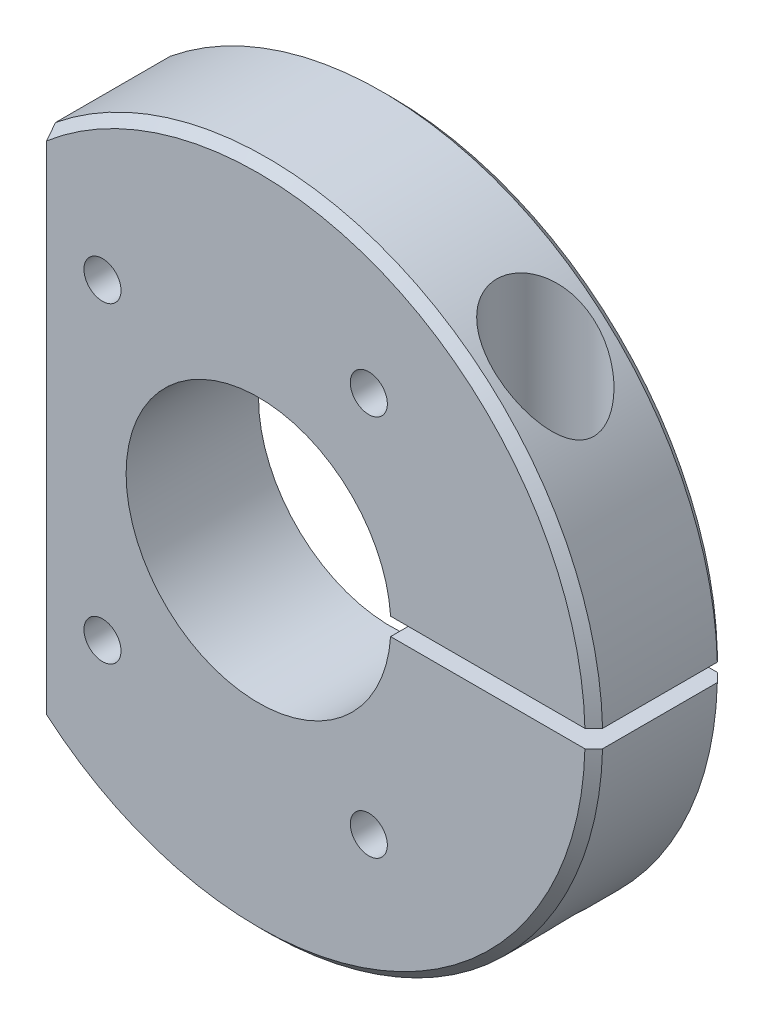
SolidWorks part; units mm, degrees
ref_plane "前视基准面" through (0, 0, 0) normal (0, 0, 1) x (1, 0, 0)
ref_plane "上视基准面" through (0, 0, 0) normal (0, 1, 0) x (1, 0, 0)
ref_plane "右视基准面" through (0, 0, 0) normal (1, 0, 0) x (0, 0, -1)
ref_plane "基准面4" through (0, 0, -7.5) normal (0, 0, -1) x (-1, 0, 0)
sketch "草图1" plane through (0, 0, -7.5) normal (0, 0, -1) x (-1, 0, 0)
  line L0 (24, -29.4618) -> (24, 29.4618)
  arc A0 (24, 29.4618) -> (24, -29.4618) centre (0, 0) ccw
extrude "凸台-拉伸1" add sketch "草图1" against normal blind 15
sketch "草图2" plane through (0, 0, 7.5) normal (0, 0, 1) x (1, 0, 0)
  line L0 (37.9868, 1) -> (14.9666, 1)
  line L1 (14.9666, -1) -> (37.9868, -1)
  arc A0 (37.9868, -1) -> (37.9868, 1) centre (0, 0) ccw
  arc A1 (14.9666, 1) -> (14.9666, -1) centre (0, 0) cw
extrude "切除-拉伸1" cut sketch "草图2" against normal through all
ref_plane "基准面5" through (0, 0, 0) normal (0, -1, 0) x (1, 0, 0)
sketch "草图3" plane through (0, 0, 0) normal (0, -1, 0) x (1, 0, 0)
  line L0 (15, 7.5) -> (0, 7.5)
  line L1 (0, 7.5) -> (0, -7.5)
  line L2 (0, -7.5) -> (15, -7.5)
  line L3 (15, -7.5) -> (15, 7.5)
  line L4 (0, 7.5) -> (0, -7.5) construction
revolve "切除-旋转1" cut sketch "草图3" angle 360 about L4
hole_wizard "Ø4.2 (4.2) 直径孔1" positions "草图5" profile "草图4" hole size "Ø4.2" standard "ANSI Metric"
sketch "草图5" plane through (0, 0, 7.5) normal (0, 0, 1) x (1, 0, 0)
  point P0 (-17.6777, -17.6777)
  point P1 (-17.6777, 17.6777)
  point P2 (12.5, 21.6506)
  point P3 (12.5, -21.6506)
sketch "草图4" plane through (-17.6777, -17.6777, 7.5) normal (1, 0, 0) x (0, -1, 0)
  line L0 (0, 0) -> (0, 15)
  line L1 (0, 15) -> (2.1, 15)
  line L2 (2.1, 15) -> (2.1, 0)
  line L5 (2.1, 0) -> (0, 0)
  line L11 (0, -6.35) -> (0, 107.95) construction
  dimension "通孔孔直径" = 4.2
  dimension "通孔孔深度" = 15
hole_wizard "Ø5.0 (5) 直径孔1" positions "草图7" profile "草图6" hole size "Ø5.0" standard "ANSI Metric"
sketch "草图7" plane through (0, -1, 0) normal (0, 1, 0) x (1, 0, 0)
  point P0 (25, 0)
sketch "草图6" plane through (25, -1, 0) normal (1, 0, 0) x (0, 0, 1)
  line L0 (0, 0) -> (0, 37)
  line L1 (0, 37) -> (2.5, 37)
  line L2 (2.5, 37) -> (2.5, 0)
  line L5 (2.5, 0) -> (0, 0)
  line L11 (0, -6.35) -> (0, 107.95) construction
  dimension "通孔孔直径" = 5
  dimension "通孔孔深度" = 37
ref_plane "基准面6" through (0, 32.6152, 0) normal (0, 1, 0) x (1, 0, 0)
hole_wizard "M6 六角头螺栓的柱形沉头孔1" positions "草图9" profile "草图8" counterbore size "M6" standard "ANSI Metric"
sketch "草图9" plane through (0, 32.6152, 0) normal (0, 1, 0) x (1, 0, 0)
  point P0 (25, 0)
sketch "草图8" plane through (25, 32.6152, 0) normal (1, 0, 0) x (0, 0, 1)
  line L0 (0, 0) -> (0, 70.6152)
  line L1 (0, 70.6152) -> (3.25, 70.6152)
  line L3 (3.25, 70.6152) -> (3.25, 24.6152)
  line L4 (3.25, 24.6152) -> (5.5, 24.6152)
  line L5 (5.5, 24.6152) -> (5.5, 0)
  line L7 (5.5, 0) -> (0, 0)
  line L11 (0, -6.35) -> (0, 107.95) construction
  dimension "通孔孔直径" = 6.5
  dimension "通孔孔深度" = 70.6152
  dimension "柱形沉头孔直径" = 11
  dimension "柱形沉头孔深度" = 24.6152
chamfer "倒角1" distance 1 angle 45 4 edges at (15.8564, -34.5337, -7.5) (15.8564, 34.5337, 7.5) (15.8564, 34.5337, -7.5) (15.8564, -34.5337, 7.5)
